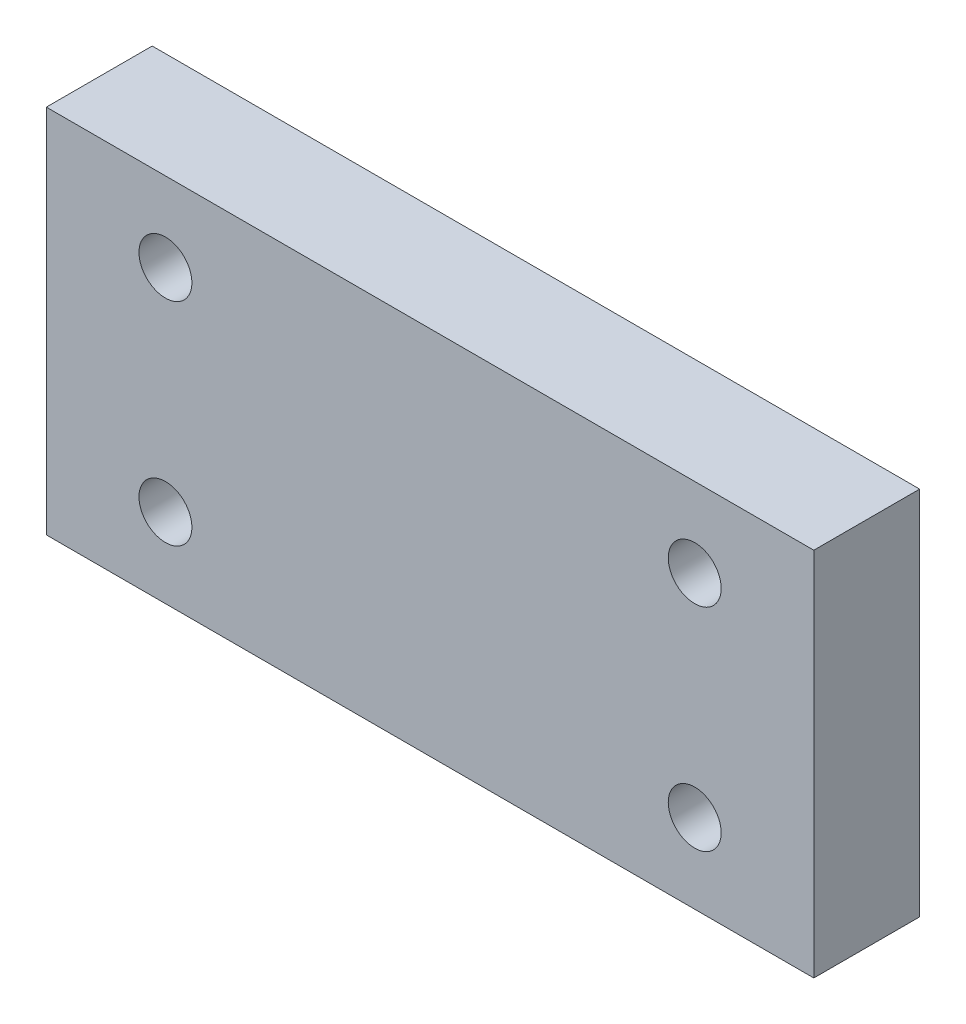
SolidWorks part; units mm, degrees
ref_plane "Front Plane" through (0, 0, 0) normal (0, 0, 1) x (1, 0, 0)
ref_plane "Top Plane" through (0, 0, 0) normal (0, 1, 0) x (1, 0, 0)
ref_plane "Right Plane" through (0, 0, 0) normal (1, 0, 0) x (0, 0, -1)
sketch "Sketch1" plane through (0, 0, 0) normal (0, 0, 1) x (1, 0, 0)
  line L0 (-291.2707, 0) -> (248.6612, 0) construction
  line L1 (145, 70) -> (-145, 70)
  line L2 (145, 70) -> (145, -70)
  line L3 (145, -70) -> (-145, -70)
  line L4 (-145, 70) -> (-145, -70)
  line L5 (145, 70) -> (-145, -70) construction
  line L6 (145, -70) -> (-145, 70) construction
  circle A0 centre (-100, 40) radius 10
  circle A1 centre (100, 40) radius 10
  circle A2 centre (100, -40) radius 10
  circle A3 centre (-100, -40) radius 10
  point P0 (0, 0)
  dimension "D3" = 20
  dimension "D4" = 20
  dimension "D1" = 140
  dimension "D2" = 290
  dimension "D5" = 45
  dimension "D6" = 30
  dimension "D7" = 30
  dimension "D8" = 45
extrude "Boss-Extrude1" add sketch "Sketch1" along normal blind 40
